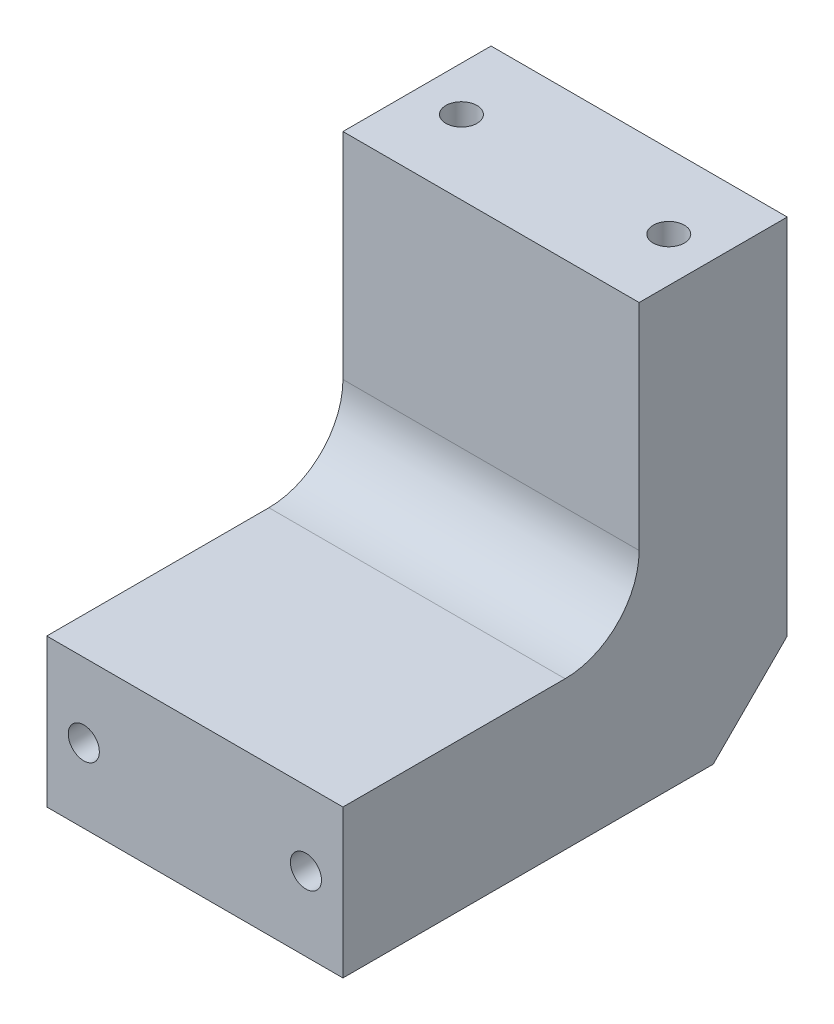
SolidWorks part; units mm, degrees
ref_plane "Front Plane" through (0, 0, 0) normal (0, 0, 1) x (1, 0, 0)
ref_plane "Top Plane" through (0, 0, 0) normal (0, 1, 0) x (1, 0, 0)
ref_plane "Right Plane" through (0, 0, 0) normal (1, 0, 0) x (0, 0, -1)
sketch "Sketch1" plane through (0, 0, 0) normal (0, 1, 0) x (1, 0, 0)
  line L1 (-20, 30) -> (20, 30)
  line L2 (-20, 30) -> (-20, -30)
  line L3 (-20, -30) -> (20, -30)
  line L4 (20, 30) -> (20, -30)
  line L5 (-20, 30) -> (20, -30) construction
  line L6 (-20, -30) -> (20, 30) construction
  point P0 (0, 0)
  dimension "D1" = 40
  dimension "D2" = 60
extrude "Boss-Extrude1" add sketch "Sketch1" along normal blind 59
sketch "Sketch2" plane through (20, 0, 0) normal (1, 0, 0) x (0, 0, -1)
  line L0 (30, 59) -> (30, 0) construction
  line L1 (-30, 59) -> (10, 59)
  line L2 (-30, 59) -> (-30, 20)
  line L3 (-30, 20) -> (10, 20)
  line L4 (10, 59) -> (10, 20)
  line L5 (-30, 0) -> (30, 0) construction
  dimension "D1" = 20
  dimension "D2" = 20
extrude "Cut-Extrude1" cut sketch "Sketch2" against normal blind 45
chamfer "Chamfer1" distance 10 angle 45 1 edges at (0, 0, -30)
fillet "Fillet1" radius 10 1 edges at (0, 20, -10)
sketch "Sketch4" plane through (0, 59, 0) normal (0, 1, 0) x (1, 0, 0)
  line L0 (0, 0) -> (0, 50000) construction
  line L1 (-20, 20) -> (49980, 20) construction
  line L2 (-20, 30) -> (-20, 10) construction
  point P7 (-20, 20)
  point P8 (-14, 20)
  point P9 (14, 20)
  dimension "D1" = 28
hole_wizard "M5 Tapped Hole1" positions "3DSketch1" profile "Sketch5" tap size "M5" standard "Gb"
sketch3d "3DSketch1"
  point P0 (-14, 59, -20)
  point P3 (14, 59, -20)
sketch "Sketch5" plane through (-14, 59, -20) normal (1, 0, 0) x (0, 0, 1)
  line L0 (0, 0) -> (0, 13.6618)
  line L1 (0, 13.6618) -> (2.1, 12.4)
  line L2 (2.1, 12.4) -> (2.1, 0)
  line L5 (2.1, 0) -> (0, 0)
  line L10 (0, 13.6618) -> (-2.1, 12.4) construction
  line L11 (0, -6.35) -> (0, 107.95) construction
  dimension "螺纹孔钻头直径" = 4.2
  dimension "螺纹孔钻头深度" = 12.4
  dimension "导头角度" = 118
cosmetic thread "Cosmetic Thread1" parameters "D1"=10, "D2"=5
cosmetic thread "Cosmetic Thread2" parameters "D1"=10, "D2"=5
sketch "Sketch6" plane through (0, 0, 30) normal (0, 0, 1) x (1, 0, 0)
  line L0 (0, 48) -> (0, -49952) construction
  line L1 (20, 59) -> (-20, 59) construction
  line L2 (20, 10) -> (-49980, 10) construction
  line L3 (20, 20) -> (20, 0) construction
  point P4 (0, 59)
  point P9 (20, 10)
  point P10 (-15, 10)
  point P11 (15, 10)
  dimension "D1" = 30
hole_wizard "M5 Tapped Hole2" positions "3DSketch2" profile "Sketch7" tap size "M5" standard "Gb"
sketch3d "3DSketch2"
  point P0 (-15, 10, 30)
  point P3 (15, 10, 30)
sketch "Sketch7" plane through (-15, 10, 30) normal (1, 0, 0) x (0, -1, 0)
  line L0 (0, 0) -> (0, 13.6618)
  line L1 (0, 13.6618) -> (2.1, 12.4)
  line L2 (2.1, 12.4) -> (2.1, 0)
  line L5 (2.1, 0) -> (0, 0)
  line L10 (0, 13.6618) -> (-2.1, 12.4) construction
  line L11 (0, -6.35) -> (0, 107.95) construction
  dimension "螺纹孔钻头直径" = 4.2
  dimension "螺纹孔钻头深度" = 12.4
  dimension "导头角度" = 118
cosmetic thread "Cosmetic Thread3" parameters "D1"=10, "D2"=5
cosmetic thread "Cosmetic Thread4" parameters "D1"=10, "D2"=5
